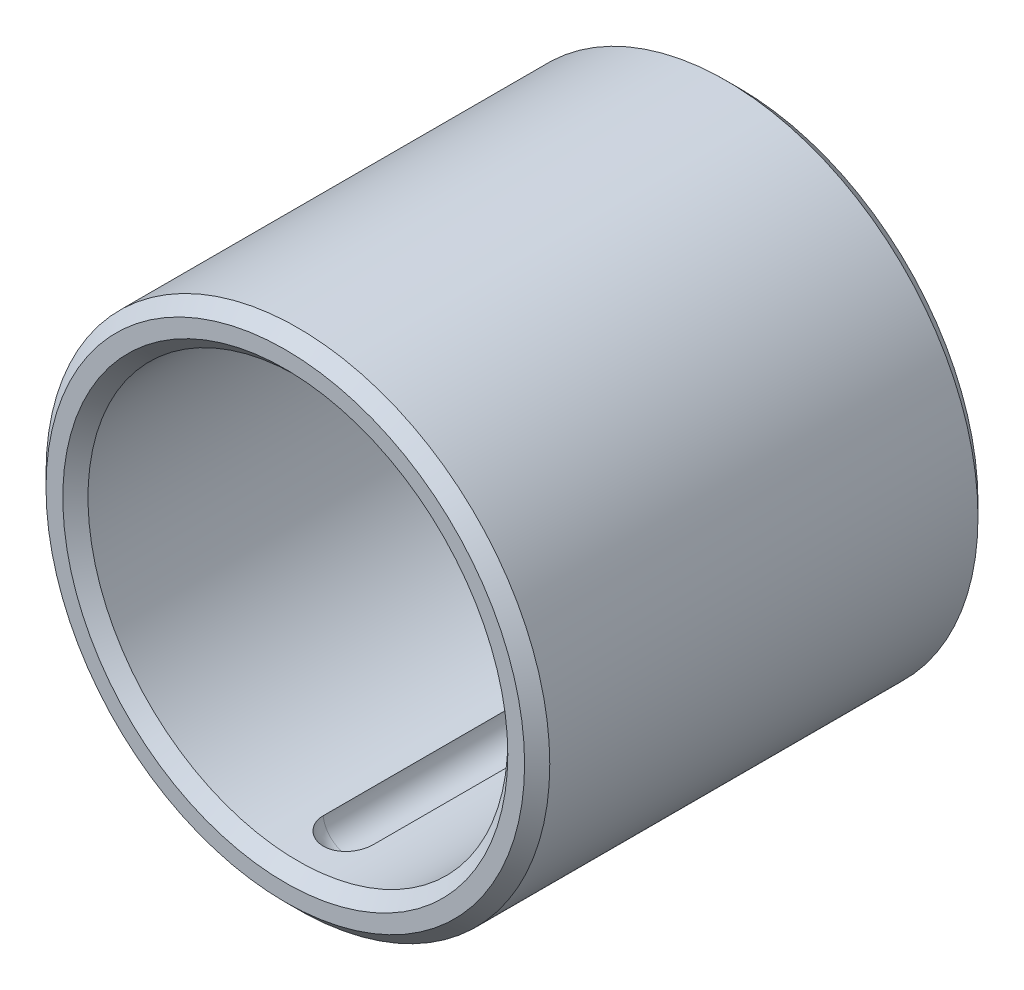
SolidWorks part; units mm, degrees
material "ZCuSn10Pb5"
ref_plane "Front Plane" through (0, 0, 0) normal (0, 0, 1) x (1, 0, 0)
ref_plane "Top Plane" through (0, 0, 0) normal (0, 1, 0) x (1, 0, 0)
ref_plane "Right Plane" through (0, 0, 0) normal (1, 0, 0) x (0, 0, -1)
sketch "Sketch1" plane through (0, 0, 0) normal (0, 0, 1) x (1, 0, 0)
  circle A0 centre (0, 0) radius 25
  circle A1 centre (0, 0) radius 30
  dimension "D1" = 60
  dimension "D2" = 50
extrude "Boss-Extrude1" add sketch "Sketch1" along normal mid plane 54
chamfer "Chamfer1" distance 1.5 angle 45 4 edges at (25, 0, -27) (30, 0, -27) (30, 0, 27) (25, 0, 27)
sketch "Sketch3" plane through (0, 0, 0) normal (1, 0, 0) x (0, 0, -1)
  line L0 (-27, 28.5) -> (-27, -28.5) construction
  line L1 (-27, 28.5) -> (-27, -28.5) construction
  line L2 (-37.9196, -27.5) -> (32.7434, -27.5) construction
  line L3 (-44.6897, 0) -> (34.2244, 0) construction
  line L4 (-22.5, 28.1827) -> (-22.5, -28.8173) construction
  line L5 (-19.5, -21.5) -> (-19.5, -27.5)
  arc A0 (-19.5, -21.5) -> (-19.5, -27.5) centre (-19.5, -24.5) ccw
  dimension "D3" = 3
  dimension "D1" = 27.5
  dimension "D2" = 4.5
  dimension "D5" = 3
  dimension "D6" = 3
revolve "Cut-Revolve10" cut sketch "Sketch3" angle 360 about L5
sketch "Sketch2" plane through (0, 0, -27) normal (0, 0, -1) x (-1, 0, 0)
  line L0 (-34.4074, 0) -> (34.7832, 0) construction
  line L1 (0, 33.5882) -> (0, -35.1163) construction
  line L2 (-30.9506, -27.5) -> (41.0011, -27.5) construction
  circle A0 centre (0, 0) radius 25 construction
  circle A1 centre (0, 0) radius 25 construction
  circle A2 centre (0, -24.5) radius 3
  dimension "D2" = 6
  dimension "D1" = 27.5
extrude "Cut-Extrude1" cut sketch "Sketch2" against normal up to next
